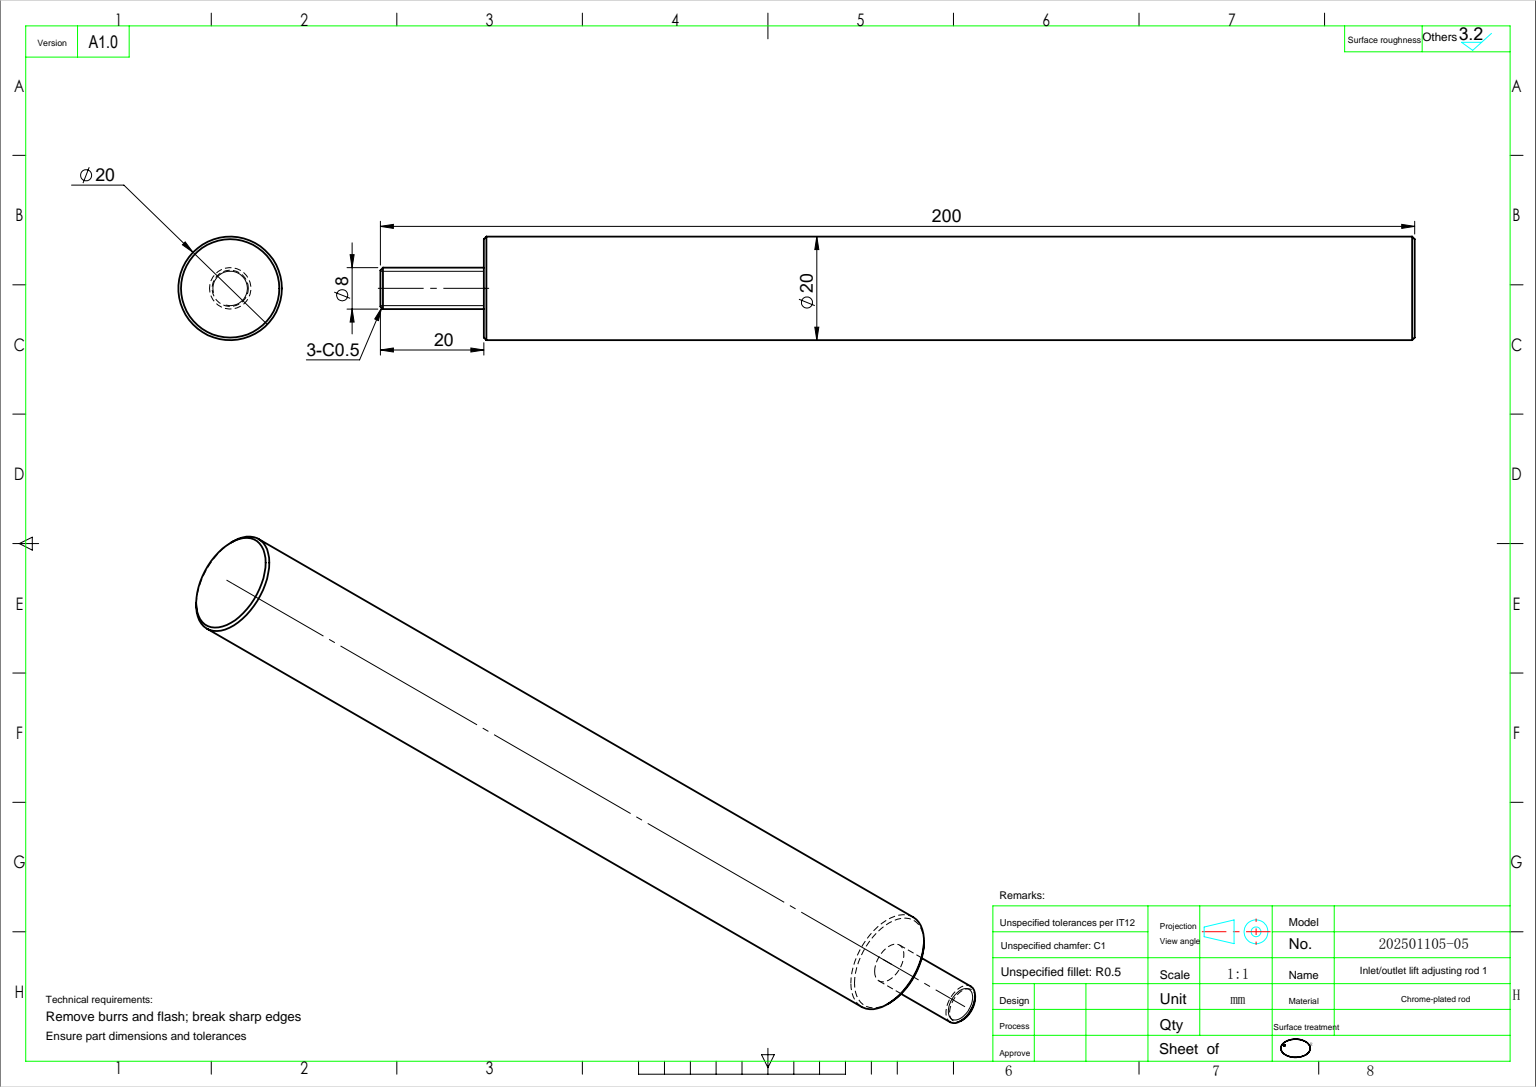
from build123d import *

# Parameters (mm, degrees)
SKETCH_1_R          = 10
EXTRUDE_1_DEPTH     = 200
SKETCH_2_OUTSIDE_W  = 62.398
SKETCH_2_OUTSIDE_H  = 62.398
SKETCH_2_OUTSIDE_R  = 4
CUT_EXTRUDE_1_DEPTH = 20
CHAMFER_1_SIZE      = 0.5


with BuildPart() as part:
    # 草图1 → 凸台-拉伸1 (new body)
    with BuildSketch(Plane.XY):
        Circle(SKETCH_1_R)
    extrude(amount=EXTRUDE_1_DEPTH)

    # 草图2 outside → 切除-拉伸1 (cut)
    with BuildSketch(Plane(origin=(0, 0, 0), x_dir=(-1, 0, 0), z_dir=(0, 0, -1))):
        Rectangle(SKETCH_2_OUTSIDE_W, SKETCH_2_OUTSIDE_H)
        Circle(SKETCH_2_OUTSIDE_R, mode=Mode.SUBTRACT)
    extrude(amount=-CUT_EXTRUDE_1_DEPTH, mode=Mode.SUBTRACT)

    # 倒角1
    chamfer_1_edges = [part.edges().sort_by_distance(p)[0] for p in [
        (4, 0, 0),
        (-10, 0, 200),
        (-10, 0, 20),
    ]]
    chamfer(chamfer_1_edges, length=CHAMFER_1_SIZE)


solid = part.part
